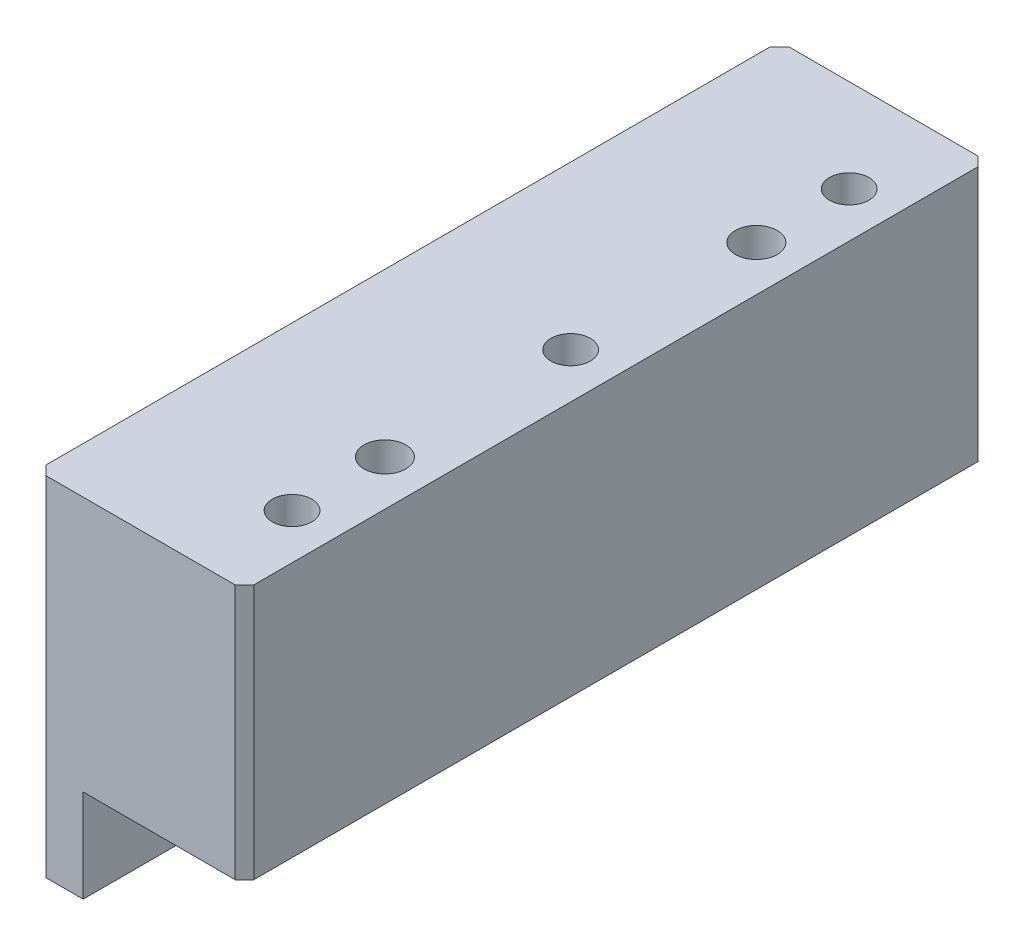
SolidWorks part; units mm, degrees
ref_plane "Front Plane" through (0, 0, 0) normal (0, 0, 1) x (1, 0, 0)
ref_plane "Top Plane" through (0, 0, 0) normal (0, 1, 0) x (1, 0, 0)
ref_plane "Right Plane" through (0, 0, 0) normal (1, 0, 0) x (0, 0, -1)
sketch "Sketch1" plane through (0, 0, 0) normal (0, 1, 0) x (1, 0, 0)
  line L1 (-22.375, 80) -> (22.375, 80)
  line L2 (-22.375, 80) -> (-22.375, -80)
  line L3 (-22.375, -80) -> (22.375, -80)
  line L4 (22.375, 80) -> (22.375, -80)
  line L5 (-22.375, 80) -> (22.375, -80) construction
  line L6 (-22.375, -80) -> (22.375, 80) construction
  point P0 (0, 0)
  dimension "D1" = 44.75
  dimension "D2" = 160
extrude "Boss-Extrude1" add sketch "Sketch1" along normal blind 75
sketch "Sketch5" plane through (0, 0, 0) normal (0, -1, 0) x (1, 0, 0)
  line L0 (22.375, -80) -> (-22.375, -80) construction
  line L1 (22.375, 80) -> (-12.375, 80)
  line L2 (22.375, 80) -> (22.375, -80)
  line L3 (22.375, -80) -> (-12.375, -80)
  line L4 (-12.375, 80) -> (-12.375, -80)
  line L5 (-22.375, -80) -> (-22.375, 80) construction
  dimension "D1" = 10
extrude "Cut-Extrude3" cut sketch "Sketch5" against normal blind 20
hole_wizard "Ø8.5 (8.5) Diameter Hole1" positions "Sketch7" profile "Sketch6" hole size "Ø8.5" standard "Gb" end condition through all
sketch "Sketch7" plane through (0, 75, 0) normal (0, 1, 0) x (-1, 0, 0)
  point P0 (-12.625, -60)
  point P3 (-12.625, 0)
  point P6 (-12.625, 60)
sketch "Sketch6" plane through (12.625, 75, -60) normal (1, 0, 0) x (0, 0, 1)
  line L0 (0, 0) -> (0, 75)
  line L1 (0, 75) -> (4.25, 75)
  line L2 (4.25, 75) -> (4.25, 0)
  line L5 (4.25, 0) -> (0, 0)
  line L11 (0, -6.35) -> (0, 107.95) construction
  dimension "通孔孔直径" = 8.5
  dimension "通孔孔深度" = 75
chamfer "Chamfer2" distance 2 angle 45 4 edges at (-22.375, 37.5, 80) (22.375, 47.5, 80) (22.375, 47.5, -80) (-22.375, 37.5, -80)
hole_wizard "CBORE for M8 Hex Socket Head Cap Screw1" positions "Sketch9" profile "Sketch8" counterbore size "M8" standard "Iso" end condition through all
sketch "Sketch9" plane through (0, 20, 0) normal (0, -1, 0) x (1, 0, 0)
  line L0 (12.625, 60) -> (12.625, 0) construction
  line L3 (0, 0) -> (32.1679, 0) construction
  point P0 (12.625, 40)
  point P2 (12.625, -40)
  dimension "D1" = 80
sketch "Sketch8" plane through (12.625, 20, 40) normal (1, 0, 0) x (0, 0, -1)
  line L0 (0, 0) -> (0, 55)
  line L1 (0, 55) -> (4.5, 55)
  line L3 (4.5, 55) -> (4.5, 40)
  line L4 (4.5, 40) -> (7.5, 40)
  line L5 (7.5, 40) -> (7.5, 0)
  line L7 (7.5, 0) -> (0, 0)
  line L11 (0, -6.35) -> (0, 107.95) construction
  dimension "通孔孔直径" = 9
  dimension "通孔孔深度" = 55
  dimension "柱形沉头孔直径" = 15
  dimension "柱形沉头孔深度" = 40
